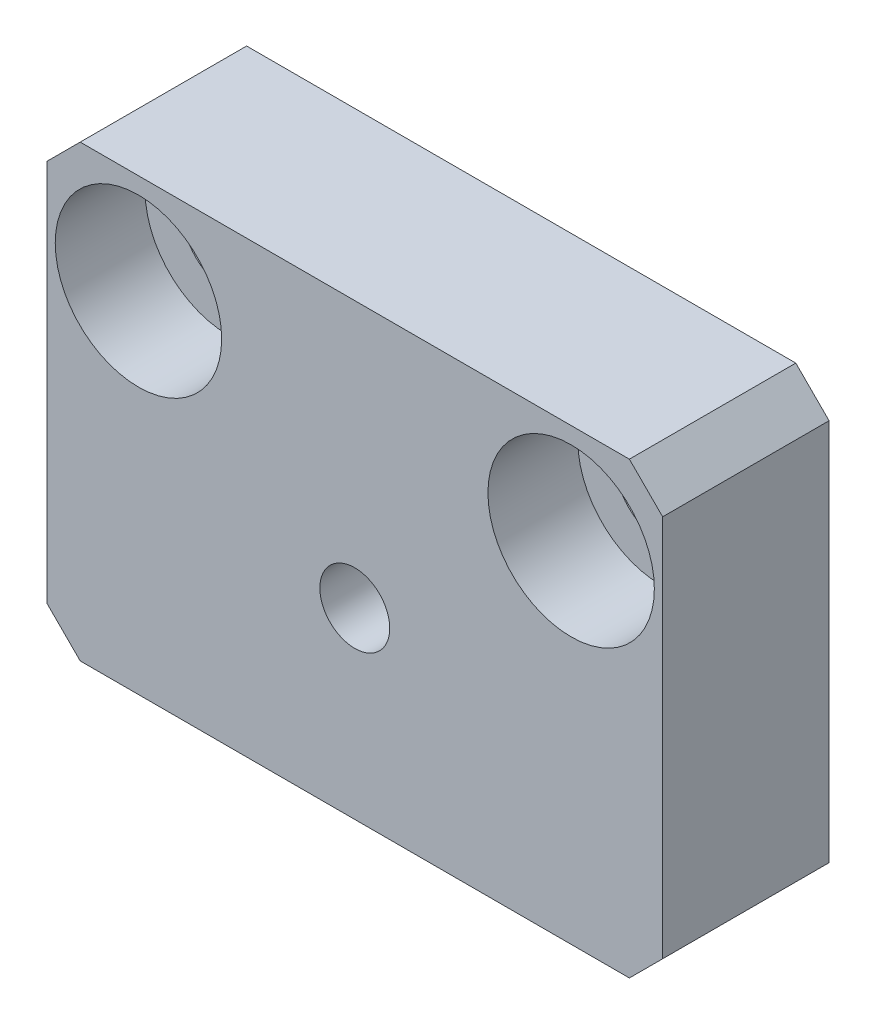
from build123d import *

# Parameters (mm, degrees)
SKETCH1_W                                           = 37
SKETCH1_H                                           = 27
BOSS_EXTRUDE1_DEPTH                                 = 10
CBORE_FOR_M5_HEX_SOCKET_HEAD_CAP_SCREW1_D           = 5.5
CBORE_FOR_M5_HEX_SOCKET_HEAD_CAP_SCREW1_CBORE_D     = 10
CBORE_FOR_M5_HEX_SOCKET_HEAD_CAP_SCREW1_CBORE_DEPTH = 5.4
M5_TAPPED_HOLE1_D                                   = 4.2
M5_TAPPED_HOLE1_DEPTH                               = 12.4
M5_TAPPED_HOLE1_TIP                                 = 1.2618073
CHAMFER1_SIZE                                       = 2


with BuildPart() as part:
    # Sketch1 → Boss-Extrude1 (new body)
    with BuildSketch(Plane.XY):
        Rectangle(SKETCH1_W, SKETCH1_H)
    extrude(amount=BOSS_EXTRUDE1_DEPTH)

    # CBORE for M5 Hex Socket Head Cap Screw1 (through all)
    with Locations(Plane.XY.offset(10)):
        with Locations((-13, 7.5), (13, 7.5)):
            CounterBoreHole(CBORE_FOR_M5_HEX_SOCKET_HEAD_CAP_SCREW1_D / 2, CBORE_FOR_M5_HEX_SOCKET_HEAD_CAP_SCREW1_CBORE_D / 2, CBORE_FOR_M5_HEX_SOCKET_HEAD_CAP_SCREW1_CBORE_DEPTH)

    # M5 Tapped Hole1
    with Locations(Plane.XY.offset(10)):
        with Locations((0, -2.5)):
            Hole(M5_TAPPED_HOLE1_D / 2, depth=M5_TAPPED_HOLE1_DEPTH)
            with Locations((0, 0, -(M5_TAPPED_HOLE1_DEPTH + M5_TAPPED_HOLE1_TIP / 2))):  # 118° drill point
                Cone(0, M5_TAPPED_HOLE1_D / 2, M5_TAPPED_HOLE1_TIP, mode=Mode.SUBTRACT)

    # Chamfer1
    chamfer1_edges = [part.edges().sort_by_distance(p)[0] for p in [
        (18.5, -13.5, 5),
        (-18.5, -13.5, 5),
        (-18.5, 13.5, 5),
        (18.5, 13.5, 5),
    ]]
    chamfer(chamfer1_edges, length=CHAMFER1_SIZE)


solid = part.part
